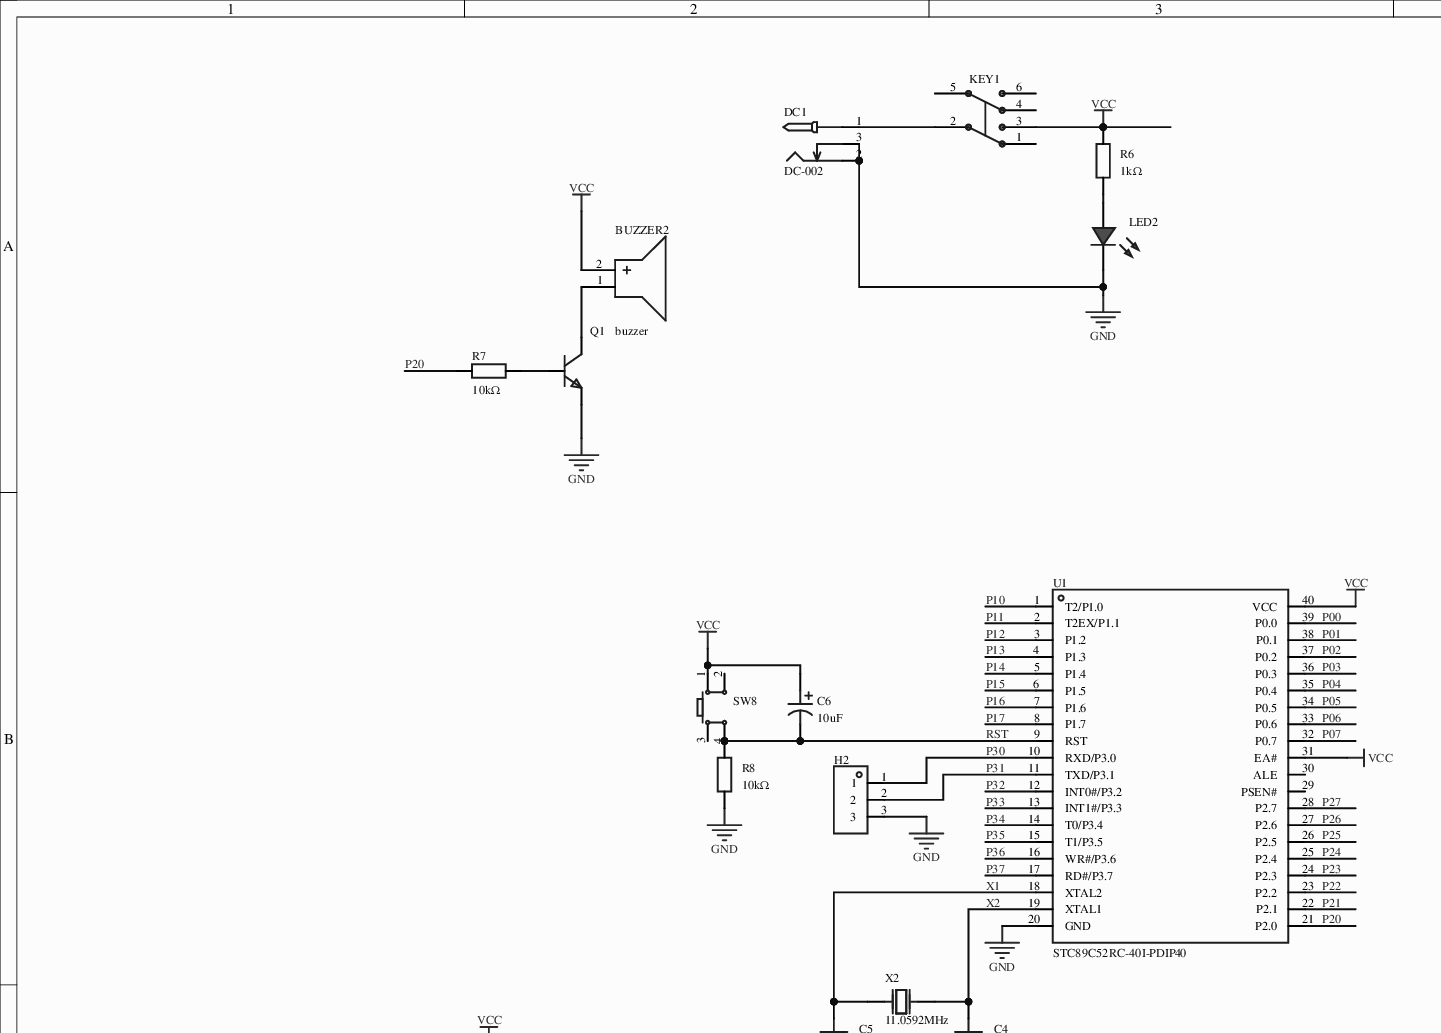
[diagram p0: MISC51000-3.schdoc, top left]
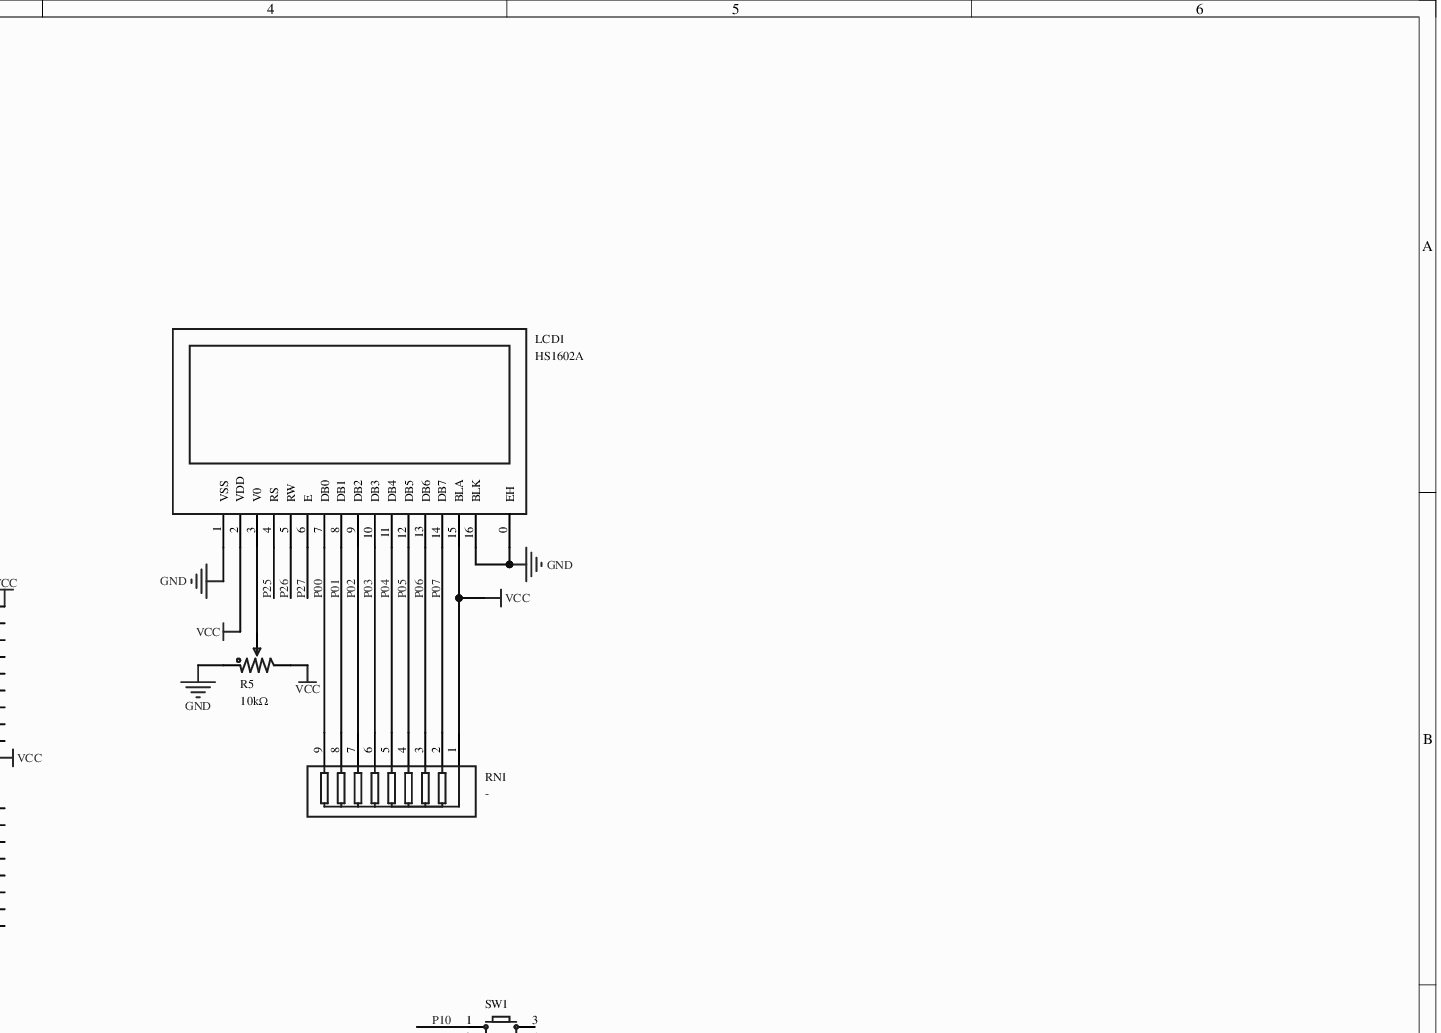
[diagram p1: MISC51000-3.schdoc, top right]
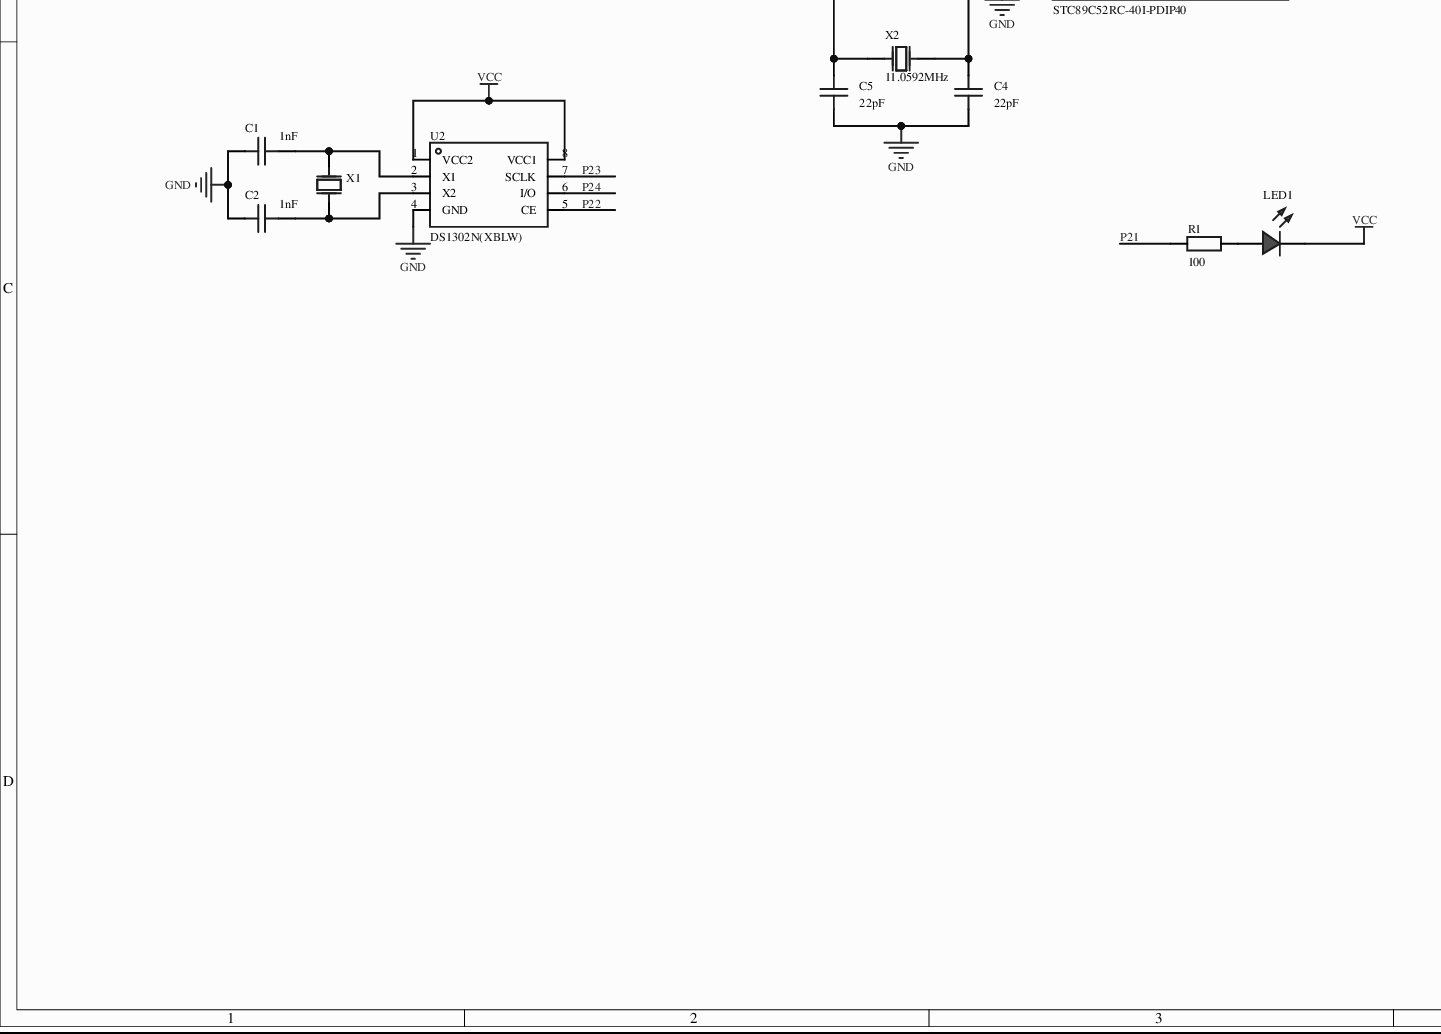
[diagram p2: MISC51000-3.schdoc, bottom left]
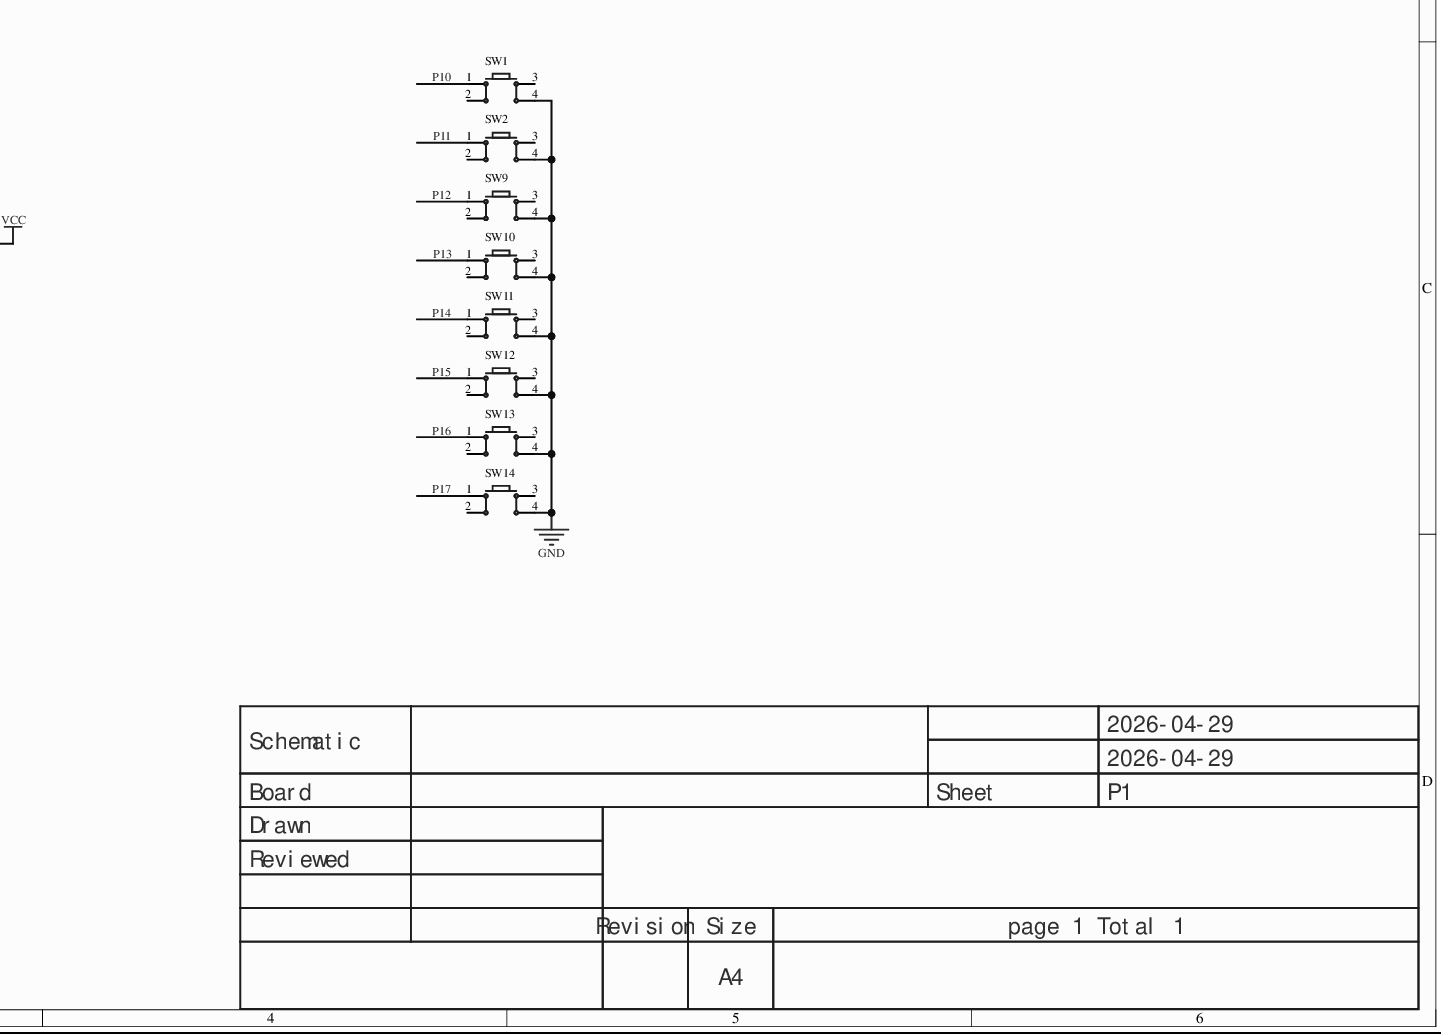
[diagram p3: MISC51000-3.schdoc, bottom right]
# Altium project MISC51000-2.PrjPcb
1 sheet, 32 parts. Net scope: global (net labels, ports and power ports of the same name join across sheets).
Board file: MISC51000.pcbdoc

## Sheet MISC51000-3.schdoc
size 420 x 297 mm; Version: V1.0; @Project Name: MISC51000; @Update Date: 2026-04-29; @Create Date: 2026-04-29; @Board Name: MISC51000; @Create Time: 10:13:01; @Page Count: 1; @Page No: 1; @Schematic Name: MISC51000; @Update Time: 10:13:01; Size: A4

### Parts
BUZZER2  buzzer  [BUZ-TH_BD12.0-P6.00-D0.9-RD]
C1  1nF  [CAP-TH_L3.8-W2.5-P2.54-D0.50]
C2  1nF  [CAP-TH_L3.8-W2.5-P2.54-D0.50]
C4  22pF  [CAP-TH_L3.8-W2.5-P2.54-D0.50]
C5  22pF  [CAP-TH_L3.8-W2.5-P2.54-D0.50]
C6  10uF  [CAP-TH_BD5.0-P2.00-D0.8-FD-10UF50VC110GL]
DC1  DC-002  [DC-IN-TH_DC-3510]
H2  (no value)  [HDR-TH_3P-P2.54-V-M]
KEY1  Non-latching switch 8.5×8.5 silent  [SW-TH_6P-L8.5-W8.5-P2.54]  (value not drawn)
LCD1  HS1602A  [LCD1602]
LED1  (no value)  [LED_TH-3mm]
LED2  (no value)  [LED_TH-3mm]
Q1  (no value)  [S8050_TO_92]
R1  100  [Res_1/8W]
R5  10kΩ  [RES-ADJ-SMD_RM065-V1]
R6  1kΩ  [Res_1/8W]
R7  10kΩ  [Res_1/8W]
R8  10kΩ  [Res_1/8W]
RN1  -  [RES-ARRAY-TH_9P-P2.54-D1.0]
SW1  (no value)  [SW-TH_4P-L6.0-W6.0-P4.50-LS6.5]
SW2  (no value)  [SW-TH_4P-L6.0-W6.0-P4.50-LS6.5]
SW8  (no value)  [SW-TH_4P-L6.0-W6.0-P4.50-LS6.5]
SW9  (no value)  [SW-TH_4P-L6.0-W6.0-P4.50-LS6.5]
SW10  (no value)  [SW-TH_4P-L6.0-W6.0-P4.50-LS6.5]
SW11  (no value)  [SW-TH_4P-L6.0-W6.0-P4.50-LS6.5]
SW12  (no value)  [SW-TH_4P-L6.0-W6.0-P4.50-LS6.5]
SW13  (no value)  [SW-TH_4P-L6.0-W6.0-P4.50-LS6.5]
SW14  (no value)  [SW-TH_4P-L6.0-W6.0-P4.50-LS6.5]
U1  STC89C52RC-40I-PDIP40  [DIP-40_L52.0-W13.7-P2.54-LS15.2-BL]
U2  DS1302N(XBLW)  [PDIP-8_L9.3-W6.4-P2.54-LS7.6-BL]
X1  11.0592MHz  [OSC-TH_L11.1-W4.7-P4.88]  (value not drawn)
X2  11.0592MHz  [OSC-TH_L11.1-W4.7-P4.88]

### Nets
GND: C1.2 C2.2 C4.1 C5.1 DC1.2 DC1.3 H2.3 LCD1.0(EH) LCD1.1(VSS) LCD1.16(BLK) LED2.2(A) Q1.1(E) R5.1 R8.1 SW1.4 SW2.4 SW9.4 SW10.4 SW11.4 SW12.4 SW13.4 SW14.4 U1.20(GND) U2.4(GND)
VCC: BUZZER2.2(+) C6.1 KEY1.3 LCD1.2(VDD) LCD1.15(BLA) LED1.2(A) R5.3 R6.2 RN1.1 SW8.1 U1.31(EA#) U1.40(VCC) U2.1(VCC2) U2.8(VCC1)
P00: LCD1.7(DB0) RN1.9 U1.39(P0.0)
P01: LCD1.8(DB1) RN1.8 U1.38(P0.1)
P02: LCD1.9(DB2) RN1.7 U1.37(P0.2)
P03: LCD1.10(DB3) RN1.6 U1.36(P0.3)
P04: LCD1.11(DB4) RN1.5 U1.35(P0.4)
P05: LCD1.12(DB5) RN1.4 U1.34(P0.5)
P06: LCD1.13(DB6) RN1.3 U1.33(P0.6)
P07: LCD1.14(DB7) RN1.2 U1.32(P0.7)
P10: SW1.1 U1.1(T2/P1.0)
P11: SW2.1 U1.2(T2EX/P1.1)
P12: SW9.1 U1.3(P1.2)
P13: SW10.1 U1.4(P1.3)
P14: SW11.1 U1.5(P1.4)
P15: SW12.1 U1.6(P1.5)
P16: SW13.1 U1.7(P1.6)
P17: SW14.1 U1.8(P1.7)
P20: R7.2 U1.21(P2.0)
P21: R1.1 U1.22(P2.1)
P22: U1.23(P2.2) U2.5(CE)
P23: U1.24(P2.3) U2.7(SCLK)
P24: U1.25(P2.4) U2.6(I/O)
P25: LCD1.4(RS) U1.26(P2.5)
P26: LCD1.5(RW) U1.27(P2.6)
P27: LCD1.6(E) U1.28(P2.7)
P30: H2.1 U1.10(RXD/P3.0)
P31: H2.2 U1.11(TXD/P3.1)
P32: U1.12(INT0#/P3.2)
P33: U1.13(INT1#/P3.3)
P34: U1.14(T0/P3.4)
P35: U1.15(T1/P3.5)
P36: U1.16(WR#/P3.6)
P37: U1.17(RD#/P3.7)
RST: C6.2 R8.2 SW8.4 U1.9(RST)
X1: C5.2 U1.18(XTAL2) X2.1(OSC1)
X2: C4.2 U1.19(XTAL1) X2.2(OSC2)
NetBUZZER2_1: BUZZER2.1(-) Q1.3(C)
NetC1_1: C1.1 U2.2(X1) X1.2(OSC2)
NetC2_1: C2.1 U2.3(X2) X1.1(OSC1)
NetDC1_1: DC1.1 KEY1.2
NetLCD1_3: LCD1.3(V0) R5.2
NetLED1_1: LED1.1(C) R1.2
NetLED2_1: LED2.1(C) R6.1
NetQ1_2: Q1.2(B) R7.1

Not connected (* = marked no-connect by the designer): KEY1 1 4 5 6; SW1 2 3; SW2 2 3; SW8 2 3; SW9 2 3; SW10 2 3; SW11 2 3; SW12 2 3; SW13 2 3; SW14 2 3; U1 29(PSEN#)* 30(ALE)*

### Notes on the sheet
- 2026-04-29
- Schematic
- Board
- Sheet
- P1
- Drawn
- Reviewed
- Revision
- Size
- A4
- page 1 Total 1

### Library data of the parts
BUZZER2 = buzzer: 3D Model: af17e4151ed84fc2a628230bf23763630819f05c4eef4c71ace90d822a990e87; 3D Model Transform: 472.44,472.176,0,270,0,0,0,0,-196.85; AddInBom: yes; Symbol: BUZZER; Device: buzzer; LCSC Part Name: buzzer; Supplier Part: C9900014030; Manufacturer Part: buzzer; Supplier Footprint: buzzer; JLCPCB Part Class: Extended Part; Supplier: LCSC; ConvertToPcb: yes; FootprintName: BUZ-TH_BD12.0-P6.00-D0.9-RD; ModelName: BUZ-TH_BD12.0-P6.00-D0.9-RD
C1 C2 C4 C5 = C315C300K3G5TA7301: Capacitance: 30pF; tolerance: ±10%; rated voltage: 25V; temperature coefficient: C0G;; Manufacturer: KEMET(基美); 3D Model: 0be8c650c9044d099e9add656cc6dda60819f05c4eef4c71ace90d822a990e87; 3D Model Transform: 149.606,98.8187,0,0,0,0,0,0,-196.85; Pin Spacing: 2.54mm; AddInBom: yes; Symbol: C315C300K3G5TA7301; Device: C315C300K3G5TA7301; LCSC Part Name: 30pF ±10% 25V; Manufacturer Part: C315C300K3G5TA7301; Supplier Footprint: 插件,P=2.54mm; JLCPCB Part Class: Extended Part; Datasheet: https://item.szlcsc.com/datasheet/C315C300K3G5TA7301/2337370.html; Supplier: LCSC; Tolerance: ±10%; Voltage Rating: 25V; Temperature Coefficient: C0G; ConvertToPcb: yes; FootprintName: CAP-TH_L3.8-W2.5-P2.54-D0.50; ModelName: CAP-TH_L3.8-W2.5-P2.54-D0.50
  C1 C2: Value: 1nF
  C4 C5: Value: 22pF
C6 = 10UF50VC110GL: Capacitance: 10uF; tolerance: ±20%; rated voltage: 50V; ripple current: 120mA@100KHz; equivalent series resistance (ESR): 1.6Ω;; Manufacturer: Econd(米朗电子); Pin Spacing: 2mm; Lifetime: 5000hrs@105℃; AddInBom: yes; Symbol: 10UF50VC110GL; Device: 10UF50VC110GL; LCSC Part Name: 10uF ±20% 50V; Supplier Part: C46867109; Manufacturer Part: 10UF50VC110GL; Supplier Footprint: 插件,D5xL11mm; JLCPCB Part Class: Extended Part; Datasheet: https://item.szlcsc.com/datasheet/10UF50VC110GL/49031974.html; Supplier: LCSC; Value: 10uF; Tolerance: ±20%; Voltage Rating: 50V; Ripple Current: 120mA@100KHz; Equivalent Series Resistance(ESR): 1.6Ω; Diameter: 5mm; Height - Seated (Max): 11mm; Operating Temperature: -40℃~+105℃; ConvertToPcb: yes; FootprintName: CAP-TH_BD5.0-P2.00-D0.8-FD-10UF50VC110GL
DC1 = DC-002: 3D Model: 28059cb5f325411c86e5e1af88d5b1310819f05c4eef4c71ace90d822a990e87; 3D Model Transform: 450.787,208.661,0,180,0,0,113.189,-47.244,-125.984; AddInBom: yes; Symbol: DC-002; Device: DC-002; LCSC Part Name: DC-002 铁脚 内铁芯1.0mm; Supplier Part: C12568; Manufacturer Part: DC-002; Supplier Footprint: 插件; JLCPCB Part Class: Extended Part; Supplier: LCSC; ConvertToPcb: yes; FootprintName: DC-IN-TH_DC-3510; ModelName: DC-IN-TH_DC-3510
H2 = HDR-M_2.54_1x3P: 3D Model: bb473b6d38ff42a99216a4fcdbdcc4cb0819f05c4eef4c71ace90d822a990e87; 3D Model Transform: 300.03877,100,0,0,0,0,0,0,-118.11; AddInBom: yes; ModelName: HDR-TH_3P-P2.54-M-LI-1X3P; Symbol: HDR-M_2.54_1x3P; Device: HDR-M_2.54_1x3P; Supplier Part: C2937625; Supplier Footprint: 插件; ConvertToPcb: yes; FootprintName: HDR-TH_3P-P2.54-V-M
KEY1 = 无自锁开关 8.5×8.5 无声: 6 pins, 8.5×8.5; Symbol: No self-locking switch 8.5×8.5 silent; 3D Model: 4c72b3966b92446eb355e1bd0fb4f8800819f05c4eef4c71ace90d822a990e87; 3D Model Transform: 342.519,334.645,0,180,0,0,0,0,-137.795; AddInBom: yes; Device: Non-latching switch 8.5×8.5 silent; LCSC Part Name: 无自锁开关 8.5×8.5  无声; Supplier Part: C26228; Manufacturer Part: 无自锁开关 8.5×8.5 无声; Supplier Footprint: 插件; JLCPCB Part Class: Extended Part; Supplier: LCSC; ConvertToPcb: yes; FootprintName: SW-TH_6P-L8.5-W8.5-P2.54; ModelName: SW-TH_6P-L8.5-W8.5-P2.54
LCD1 = HS1602A: Controller chip: SPLC780; size (inch): 2;; Manufacturer: HS(汉昇); 3D Model: f9d832f46a914cadb50fc4d4cefd25170819f05c4eef4c71ace90d822a990e87; 3D Model Transform: 3149.6,1417.32,0,0,0,0,0,0,-118.11; AddInBom: yes; Symbol: HS1602A; Device: HS1602A; LCSC Part Name: 2.0寸16*2单色字符字符液晶显示屏; Supplier Part: C5329588; Manufacturer Part: HS1602A; Supplier Footprint: -; JLCPCB Part Class: Extended Part; Datasheet: https://atta.szlcsc.com/upload/public/pdf/source/20221212/35734F14DBB323F90DD8DBE1717CD9FD.pdf; Supplier: LCSC; Main Control Chip: SPLC780; Size: 2; Operating Temperature: -20℃~+70℃; ConvertToPcb: yes; FootprintName: LCD1602; ModelName: LCD1602
LED1 LED2 = LED_TH-R_3mm: 3D Model: a497c992633541038a38947cdc58012f0819f05c4eef4c71ace90d822a990e87; 3D Model Transform: 141.274,153.327,0,0,0,0,-5.984,0,-137.795; ConvertToPcb: yes; ModelName: LED-TH-3mm_R; Symbol: LED_TH-R; Device: LED_TH-R_3mm; Supplier Footprint: 插件; AddInBom: yes; FootprintName: LED_TH-3mm
Q1 = S8050_TO_NPN: ConvertToPcb: yes; ModelId: aafe8e06f2154e7c93506efd0d6632dd0819f05c4eef4c71ace90d822a990e87; ModelName: TO-92-3_L4.9-W3.7-P1.27-L; ModelTransform: 180.78,141.44,417.3,0,0,0,0,0,-200; Symbol: S8050_TO_NPN; Device: S8050_TO_NPN; AddInBom: yes; Supplier Footprint: TO-92; FootprintName: S8050_TO_92
R1 R6-R8 = Res_AXIAL-1/8W: Symbol: Resistor; 3D Model: b2b5ae7ae4c642178fe0039925c86a3f0819f05c4eef4c71ace90d822a990e87; 3D Model Transform: 282.86,66.88,253.09,0,0,0,0,0,-191; ConvertToPcb: yes; ModelName: RES-TH_BD1.8-L3.2-P7.20-D0.4; Device: Res_AXIAL-1/8W; Supplier Footprint: 轴向引线; AddInBom: yes; FootprintName: Res_1/8W
  R1: Value: 100
  R6: Value: 1kΩ
  R7 R8: Value: 10kΩ
R5 = RM065-103(10K): Resistance: 10kΩ; tolerance: ±25%; power: 100mW;; Manufacturer: BOCHEN(博晨); 3D Model: c816c2b7942147f5a832150e8ef6960c0819f05c4eef4c71ace90d822a990e87; 3D Model Transform: 255.905,283.464,0,0,0,0,0.025,-3.937,-157.48; Voltage Rating: 50V; AddInBom: yes; Symbol: RM065-103(10K); Device: RM065-103(10K); LCSC Part Name: 10kΩ ±25%; Supplier Part: C5205021; Manufacturer Part: RM065-103(10K); Supplier Footprint: 插件,7.3x6.4mm; JLCPCB Part Class: Extended Part; Datasheet: https://item.szlcsc.com/datasheet/RM065-103(10K)/5896379.html; Supplier: LCSC; Value: 10kΩ; Tolerance: ±25%; Power(Watts): 100mW; ConvertToPcb: yes; FootprintName: RES-ADJ-SMD_RM065-V1; ModelName: RES-ADJ-SMD_RM065-V1
RN1 = 排阻 10 K 5%: Number of resistors: -; resistance: -; power per element: -;; Symbol: 10 K 5%; Device: Resistor network 10 K 5%; AddInBom: yes; ModelId: d106c67f29e14d8080ba548247a719a10819f05c4eef4c71ace90d822a990e87; ModelName: SIP-9_L22.8-W3.0-H8.5-P2.54; ModelTransform: 918.1084,118.11,0,0,0,0,0,0,-137.795; LCSC Part Name: 10KΩ (103) ±5%; SupplierPart: C26615; ManufacturerPart: 排阻 10 K 5%; Supplier Footprint: 插件; JLCPCB Part Class: Extended Part; Supplier: LCSC; ConvertToPcb: yes; FootprintName: RES-ARRAY-TH_9P-P2.54-D1.0; Number of Resistors: -; Value: -; Power(Watts): -; Number of Pins: -
SW1 SW2 SW8-SW14 = Key_TH_6x6x6: Contact current: 50mA; rated voltage (DC): 12V; insulation resistance: 100MΩ; circuit structure: SPST; mounting: through-hole; button shape: round; button/cap colour: black; actuating force: 260gf@±30gf; operating temperature: -25℃~+70℃; pin style: PC pin; switch length: 6mm; switch width: 6mm; switch height: 6mm; with bracket: no;; Symbol: Tactile switch; 3D Model: 20eee248bc684ccd8cbdbb1d0d91ec6f0819f05c4eef4c71ace90d822a990e87; 3D Model Transform: 236.22,323.03,0,90,0,0,0,0,-137.795; AddInBom: yes; ModelName: SW-TH_4P-L6.0-W6.0-H5.0-LS6.5-P4.50; Device: Key_TH_6x6x6; Supplier Footprint: 插件; ConvertToPcb: yes; FootprintName: SW-TH_4P-L6.0-W6.0-P4.50-LS6.5
U1 = STC89C52RC-40I-PDIP40: CPU core: 51 family; max CPU frequency: -;; Manufacturer: STC; AddInBom: yes; ModelId: 16d4686a009b4ddca948f91eddb57b140819f05c4eef4c71ace90d822a990e87; ModelName: DIP-40_L52.3-W13.8-H4.0-LS15.24-P2.54; ModelTransform: 2059.051,615.743,0,0,0,0,0,0,-118.11; Program Storage Size: 8KB; Program Memory Type: FLASH; Voltage - Supply: 3.3V~5.5V; Symbol: STC89C52RC-40I; Device: STC89C52RC-40I-PDIP40; LCSC Part Name: 单片机原理及应用; SupplierPart: C14022; ManufacturerPart: STC89C52RC-40I-PDIP40; Supplier Footprint: DIP-40; JLCPCB Part Class: Extended Part; Datasheet: https://item.szlcsc.com/datasheet/STC89C52RC-40I-PDIP40/14679.html; Supplier: LCSC; ConvertToPcb: yes; FootprintName: DIP-40_L52.0-W13.7-P2.54-LS15.2-BL; CPU Core: 51 family; CPU Maximum Speed: -; RAM Size: -; EEPROM: -; Number of I/O: -; ADC (Bit): -; DAC (Bit): -
U2 = DS1302N(XBLW): Interface type: Three-wire serial interface; crystal: external; alarm output: -;; Manufacturer: XBLW(芯伯乐); AddInBom: yes; ModelId: fe5fd42f66544692923c5fbf1ee41ec70819f05c4eef4c71ace90d822a990e87; ModelName: PDIP-8_L10.2-W5.9-H4.5-P2.54-LS7.6-BL; ModelTransform: 364.173,311.8104,0,0,0,0,0,0,-118.11; Voltage - Supply: 2V~5.5V; Current - Supply: 1uA; Symbol: DS1302N(XBLW); Device: DS1302N(XBLW); LCSC Part Name: DS1302N(XBLW); SupplierPart: C42395632; ManufacturerPart: DS1302N(XBLW); Supplier Footprint: DIP-8; JLCPCB Part Class: Extended Part; Datasheet: https://atta.szlcsc.com/upload/public/pdf/source/20241125/ED583BD048AAE751CB9F5E4637775452.pdf; Supplier: LCSC; ConvertToPcb: yes; FootprintName: PDIP-8_L9.3-W6.4-P2.54-LS7.6-BL; Interface: Three-wire serial interface; crystal oscillator: External; Alarm Output: -; Operating Temperature: -40℃~+85℃
X1 X2 = 9AC11059302060C3: Crystal type: through-hole crystal; frequency: 11.0592MHz; frequency tolerance at room temperature: ±20ppm; load capacitance: 30pF;; Manufacturer: JGHC(晶光华); 3D Model: f2ed30de83344a4b83b1c4b1b9fe18560819f05c4eef4c71ace90d822a990e87; 3D Model Transform: 436.37503,185.039,0,0,0,0,0,0,-137.795; Equivalent Series Resistance(ESR): 60Ω; AddInBom: yes; Symbol: 9AC11059302060C3; Device: 9AC11059302060C3; LCSC Part Name: 11.0592MHz ±20ppm 30pF; Supplier Part: C2715911; Manufacturer Part: 9AC11059302060C3; Supplier Footprint: HC-49S; JLCPCB Part Class: Extended Part; Datasheet: https://item.szlcsc.com/datasheet/9AC11059302060C3/2832137.html; Supplier: LCSC; Type: Through-hole crystal; Value: 11.0592MHz; Normal temperature Frequency Tolerance: ±20ppm; Load Capacitance: 30pF; Operating Temperature: -40℃~+85℃; ConvertToPcb: yes; FootprintName: OSC-TH_L11.1-W4.7-P4.88; ModelName: OSC-TH_L11.1-W4.7-P4.88